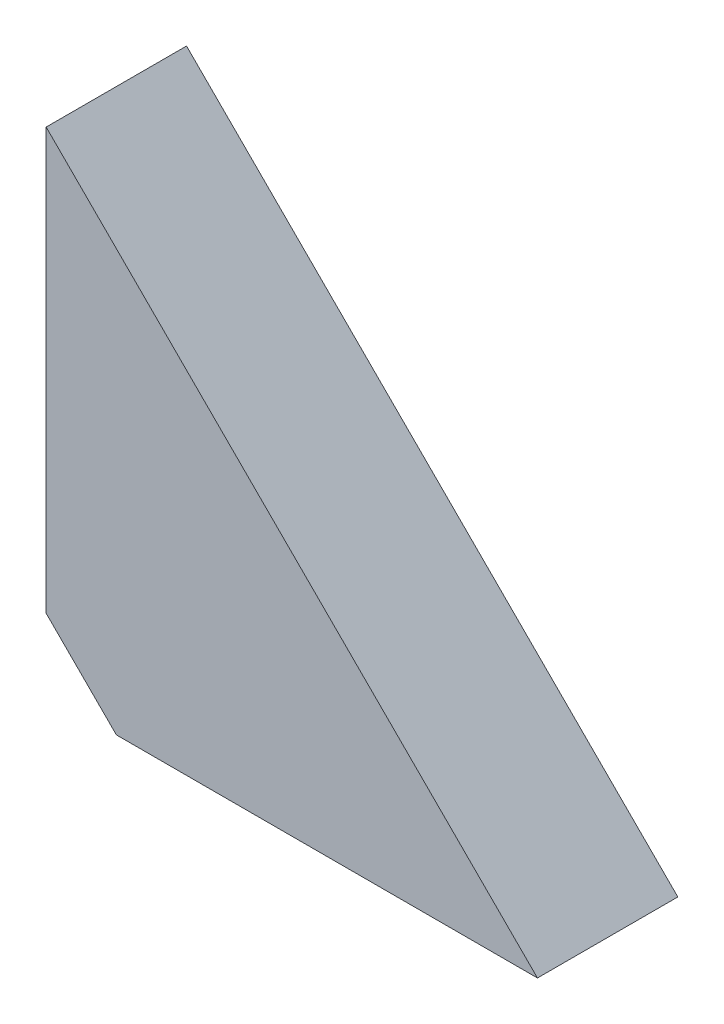
SolidWorks part; units mm, degrees
material "普通碳钢"
ref_plane "前视" through (0, 0, 0) normal (0, 0, 1) x (1, 0, 0)
ref_plane "上视" through (0, 0, 0) normal (0, 1, 0) x (1, 0, 0)
ref_plane "右视" through (0, 0, 0) normal (1, 0, 0) x (0, 0, -1)
sketch "草图1" plane through (0, 0, 0) normal (0, 0, 1) x (1, 0, 0)
  line L0 (-275.2055, 0) -> (294.863, 0) construction
  line L1 (0, 155.3425) -> (0, -166.8493) construction
  line L2 (0, 70) -> (0, 0)
  line L3 (0, 0) -> (70, 0)
  line L4 (70, 0) -> (0, 70)
  dimension "D1" = 70
  dimension "D2" = 70
extrude "凸台-拉伸1" add sketch "草图1" along normal blind 20
chamfer "倒角1" distance 10 angle 45 1 edges at (0, 0, 10)
